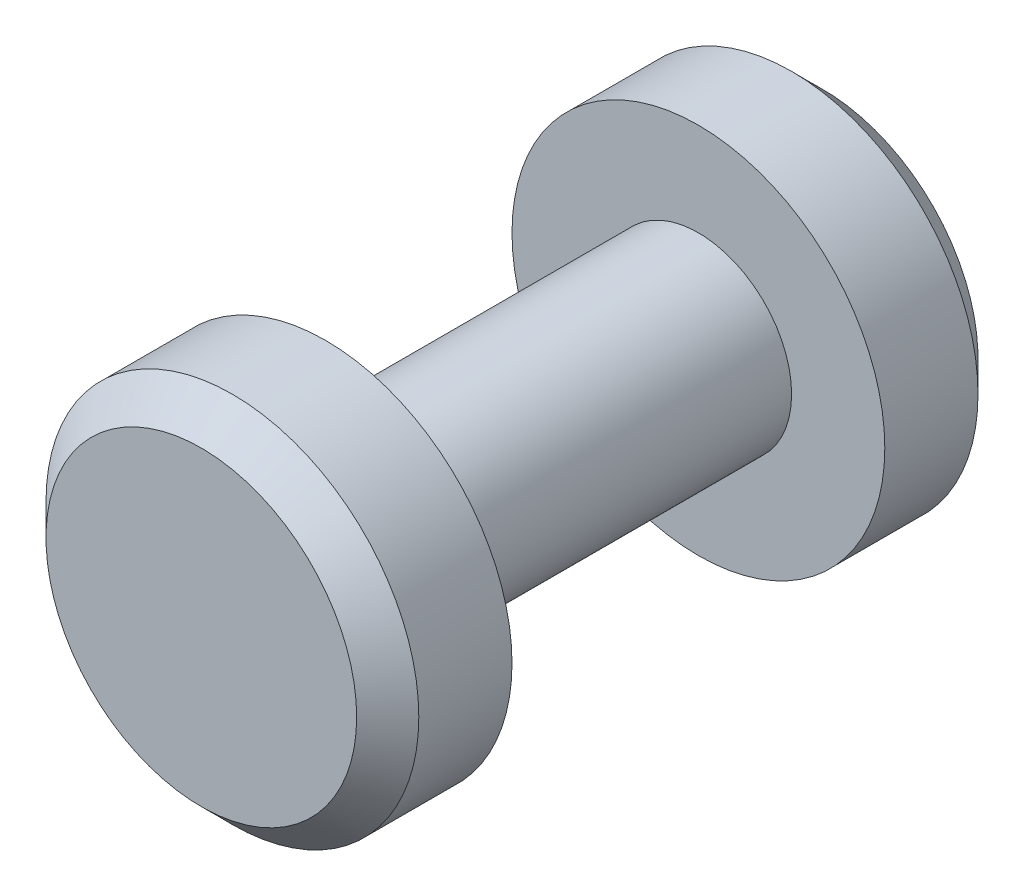
from build123d import *

# Parameters (mm, degrees)
SKETCH_1_R      = 3
EXTRUDE_1_DEPTH = 12
SKETCH_2_R      = 6
EXTRUDE_2_DEPTH = 4
CHAMFER_1_SIZE  = 1
EXTRUDE_START   = 4
SKETCH_3_R      = 6
EXTRUDE_3_DEPTH = 4
CHAMFER_2_SIZE  = 1


with BuildPart() as part:
    # 草图1 → 凸台-拉伸1 (new body)
    with BuildSketch(Plane.XY):
        Circle(SKETCH_1_R)
    extrude(amount=EXTRUDE_1_DEPTH)

    # 草图2 → 凸台-拉伸2 (add)
    with BuildSketch(Plane.XY.offset(12)):
        Circle(SKETCH_2_R)
    extrude(amount=EXTRUDE_2_DEPTH)

    # 倒角1
    chamfer_1_edges = [part.edges().sort_by_distance(p)[0] for p in [
        (-6, 0, 16),
    ]]
    chamfer(chamfer_1_edges, length=CHAMFER_1_SIZE)

    # 草图3 → 凸台-拉伸3 (add)
    with BuildSketch(Plane(origin=(0, 0, 0), x_dir=(-1, 0, 0), z_dir=(0, 0, -1)).offset(EXTRUDE_START)):
        with Locations(Location((0, 0, 0), (0, 0, 180))):
            Circle(SKETCH_3_R)
    extrude(amount=-EXTRUDE_3_DEPTH)

    # 倒角2
    chamfer_2_edges = [part.edges().sort_by_distance(p)[0] for p in [
        (-6, 0, -4),
    ]]
    chamfer(chamfer_2_edges, length=CHAMFER_2_SIZE)


solid = part.part
